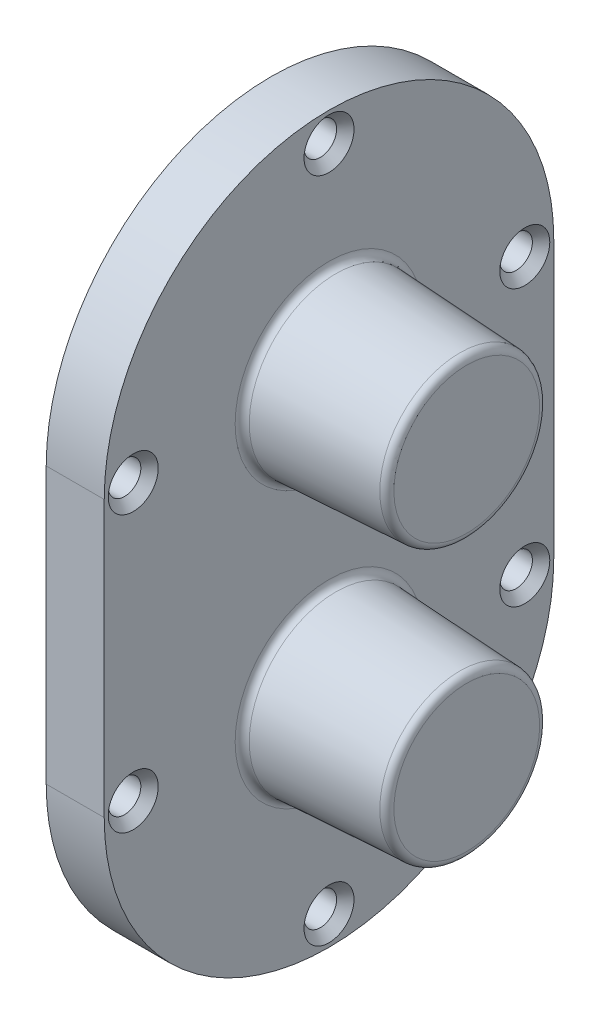
SolidWorks part; units mm, degrees
ref_plane "Front Plane" through (0, 0, 0) normal (0, 0, 1) x (1, 0, 0)
ref_plane "Top Plane" through (0, 0, 0) normal (0, 1, 0) x (1, 0, 0)
ref_plane "Right Plane" through (0, 0, 0) normal (1, 0, 0) x (0, 0, -1)
other "Configuration Table"
ref_plane "Plane1" through (8, 0, 0) normal (1, 0, 0) x (0, 0, -1)
sketch "Sketch1" plane through (8, 0, 0) normal (1, 0, 0) x (0, 0, -1)
  line L0 (31, -19) -> (31, 19)
  line L1 (-31, 19) -> (-31, -19)
  arc A0 (-31, -19) -> (31, -19) centre (0, -19) ccw
  arc A1 (31, 19) -> (-31, 19) centre (0, 19) ccw
extrude "Boss-Extrude1" add sketch "Sketch1" against normal blind 8
sketch "Sketch2" plane through (0, 0, 0) normal (0, 0, 1) x (1, 0, 0)
  line L0 (8, -7.0043) -> (8, -19)
  line L1 (8, -19) -> (27, -19)
  line L2 (27, -19) -> (27, -8)
  line L3 (27, -8) -> (8, -7.0043)
  line L4 (8, -19) -> (27, -19) construction
revolve "Revolve1" add sketch "Sketch2" angle 360 about L4
sketch "Sketch3" plane through (0, 0, 0) normal (0, 0, 1) x (1, 0, 0)
  line L0 (8, 30.9957) -> (8, 19)
  line L1 (8, 19) -> (27, 19)
  line L2 (27, 19) -> (27, 30)
  line L3 (27, 30) -> (8, 30.9957)
  line L4 (8, 19) -> (27, 19) construction
revolve "Revolve2" add sketch "Sketch3" angle 360 about L4
hole_wizard "Ø16.0 (16) Diameter Hole1" positions "Sketch5" profile "Sketch4" hole size "Ø16.0" standard "ANSI Metric"
sketch "Sketch5" plane through (0, 0, 0) normal (-1, 0, 0) x (0, 0, 1)
  point P0 (0, 19)
  point P1 (0, -19)
sketch "Sketch4" plane through (0, 19, 0) normal (0, 1, 0) x (0, 0, 1)
  line L0 (0, 0) -> (0, 24)
  line L1 (0, 24) -> (8, 24)
  line L2 (8, 24) -> (8, 0)
  line L5 (8, 0) -> (0, 0)
  line L10 (0, 24) -> (-8, 24) construction
  line L11 (0, -6.35) -> (0, 107.95) construction
  dimension "孔直径" = 16
  dimension "孔深度" = 24
  dimension "导头角度" = 180
hole_wizard "Ø4.5 (4.5) Diameter Hole1" positions "Sketch7" profile "Sketch6" hole size "Ø4.5" standard "ANSI Metric"
sketch "Sketch7" plane through (8, 0, 0) normal (1, 0, 0) x (0, 0, -1)
  point P0 (0, 46)
  point P1 (-27, 19)
  point P2 (27, 19)
  point P3 (-27, -19)
  point P4 (27, -19)
  point P5 (0, -46)
sketch "Sketch6" plane through (8, 46, 0) normal (0, 1, 0) x (0, 0, -1)
  line L0 (0, 0) -> (0, 8)
  line L1 (0, 8) -> (2.25, 8)
  line L2 (2.25, 8) -> (2.25, 0)
  line L5 (2.25, 0) -> (0, 0)
  line L11 (0, -6.35) -> (0, 107.95) construction
  dimension "通孔孔直径" = 4.5
  dimension "通孔孔深度" = 8
chamfer "Chamfer1" distance 1.2 angle 45 6 edges at (8, -19, 24.75) (8, -46, -2.25) (8, 46, -2.25) (8, 19, 24.75) (8, -19, -29.25) (8, 19, -29.25)
fillet "Fillet1" radius 1 4 edges at (27, 30, 0) (8, 19, -11.9957) (27, -19, -11) (8, -19, -11.9957)
